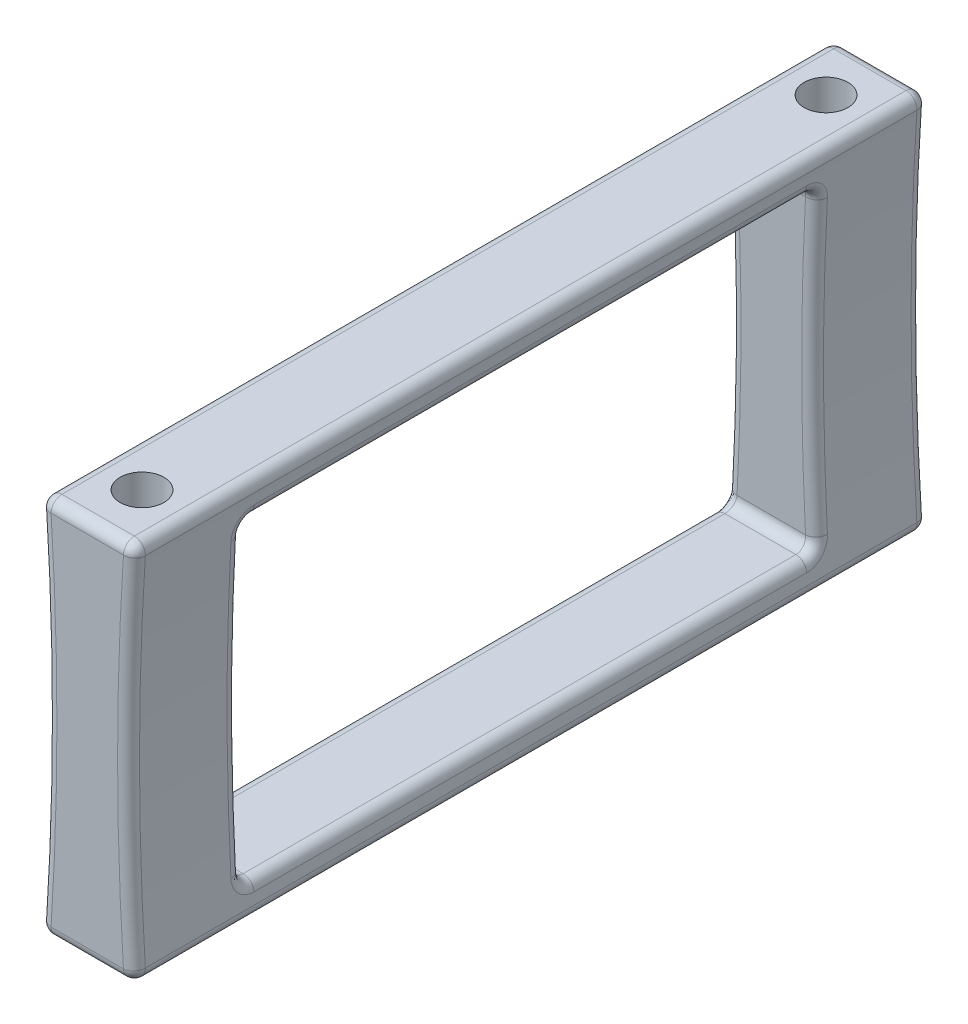
from build123d import *

# Parameters (mm, degrees)
EXTRUDE_1_DEPTH          = 58
CUT_EXTRUDE_1_DEPTH      = 60.744957946
CUT_EXTRUDE_1_DEPTH_BACK = 60.744957946
SKETCH_2_W               = 42
SKETCH_2_H               = 23
SKETCH_3_R               = 1.6
CUT_EXTRUDE_2_DEPTH      = 65.413430277
FILLET_1_R               = 0.8


with BuildPart() as part:
    # 草图1 → 凸台-拉伸1 (new body)
    with BuildSketch(Plane.XY):
        with BuildLine():
            Line((-3.5, 13.9), (3.5, 13.9))
            ThreePointArc((3.5, 13.9), (3.017556878, 0), (3.5, -13.9))
            Line((3.5, -13.9), (-3.5, -13.9))
            ThreePointArc((-3.5, -13.9), (-3.017556878, 0), (-3.5, 13.9))
        make_face()
    extrude(amount=EXTRUDE_1_DEPTH)

    # 草图2 → 切除-拉伸1 (cut, two sides: drawn at the far end of the back side and taken through both)
    with BuildSketch(Plane(origin=(0, 0, 0), x_dir=(0, 0, -1), z_dir=(1, 0, 0)).offset(-CUT_EXTRUDE_1_DEPTH_BACK)):
        with Locations((-29, 0)):
            Rectangle(SKETCH_2_W, SKETCH_2_H)
    extrude(amount=CUT_EXTRUDE_1_DEPTH + CUT_EXTRUDE_1_DEPTH_BACK, mode=Mode.SUBTRACT)

    # 草图3 → 切除-拉伸2 (cut, through all)
    with BuildSketch(Plane(origin=(0, 13.9, 0), x_dir=(1, 0, 0), z_dir=(0, 1, 0))):
        with Locations(Location((0, -4, 0), (0, 0, 180))):
            Circle(SKETCH_3_R)
        with Locations(Location((0, -54, 0), (0, 0, 180))):
            Circle(SKETCH_3_R)
    extrude(amount=-CUT_EXTRUDE_2_DEPTH, mode=Mode.SUBTRACT)

    # 圆角1
    fillet_1_edges = [part.edges().sort_by_distance(p)[0] for p in [
        (3.017556878, 0, 58),
        (3.34765802, 11.5, 29),
        (3.017556878, 0, 50),
        (3.34765802, -11.5, 29),
        (3.017556878, 0, 8),
        (0, 13.9, 58),
        (-3.017556878, 0, 8),
        (0, 11.5, 8),
        (-3.34765802, -11.5, 29),
        (0, -11.5, 8),
        (-3.017556878, 0, 50),
        (0, -11.5, 50),
        (-3.34765802, 11.5, 29),
        (0, 11.5, 50),
        (-3.017556878, 0, 58),
        (0, 13.9, 0),
        (3.017556878, 0, 0),
        (0, -13.9, 0),
        (-3.017556878, 0, 0),
        (-3.5, 13.9, 29),
        (3.5, 13.9, 29),
        (3.5, -13.9, 29),
        (-3.5, -13.9, 29),
        (0, -13.9, 58),
    ]]
    fillet(fillet_1_edges, radius=FILLET_1_R)


solid = part.part
